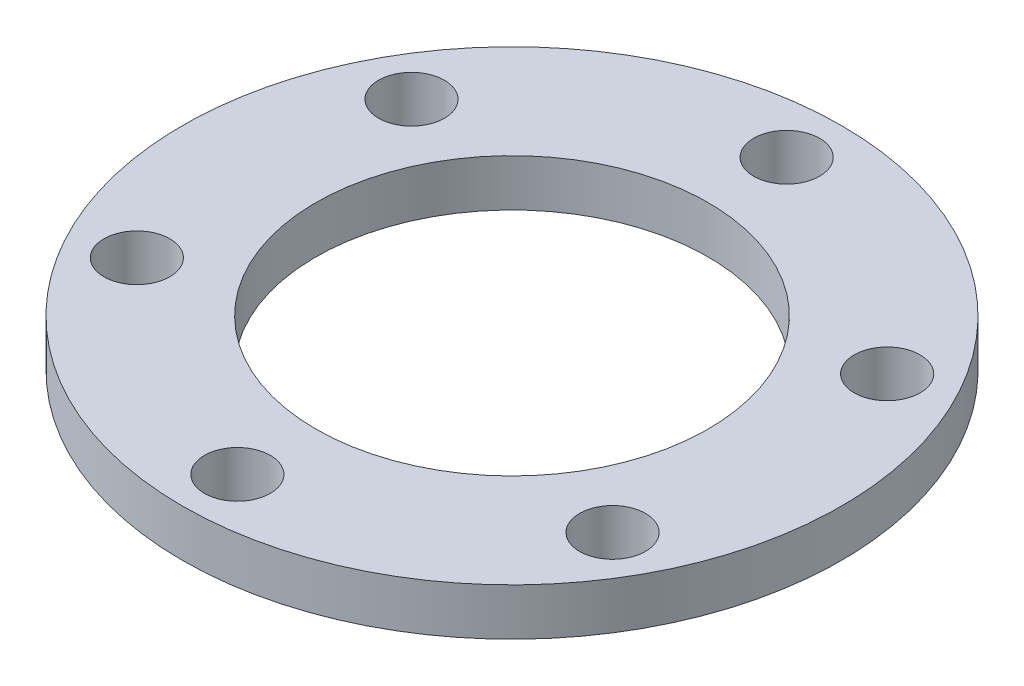
from build123d import *

# Parameters (mm, degrees)
SKETCH_1_R      = 21
SKETCH_1_R_2    = 12.5
SKETCH_1_R_3    = 2.1
EXTRUDE_1_DEPTH = 3


with BuildPart() as part:
    # 草图1 → 凸台-拉伸1 (new body)
    with BuildSketch(Plane(origin=(0, 0, 0), x_dir=(1, 0, 0), z_dir=(0, 1, 0))):
        with Locations(Location((0, 0, 0), (0, 0, 270))):
            Circle(SKETCH_1_R)
        with Locations(Location((0, 0, 0), (0, 0, 270))):
            Circle(SKETCH_1_R_2, mode=Mode.SUBTRACT)
        with Locations(Location((0, 17.5, 0), (0, 0, 270))):
            Circle(SKETCH_1_R_3, mode=Mode.SUBTRACT)
        with Locations(Location((15.155444566, 8.75, 0), (0, 0, 270))):
            Circle(SKETCH_1_R_3, mode=Mode.SUBTRACT)
        with Locations(Location((15.155444566, -8.75, 0), (0, 0, 270))):
            Circle(SKETCH_1_R_3, mode=Mode.SUBTRACT)
        with Locations(Location((0, -17.5, 0), (0, 0, 270))):
            Circle(SKETCH_1_R_3, mode=Mode.SUBTRACT)
        with Locations(Location((-15.155444566, -8.75, 0), (0, 0, 270))):
            Circle(SKETCH_1_R_3, mode=Mode.SUBTRACT)
        with Locations(Location((-15.155444566, 8.75, 0), (0, 0, 270))):
            Circle(SKETCH_1_R_3, mode=Mode.SUBTRACT)
    extrude(amount=EXTRUDE_1_DEPTH)


solid = part.part
